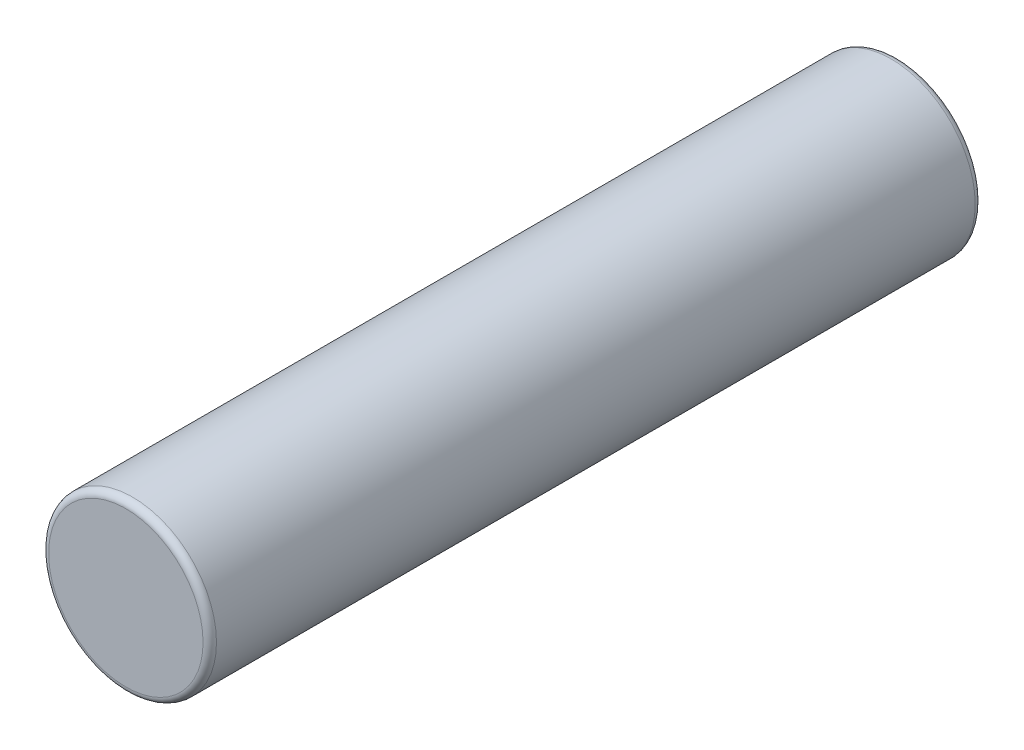
SolidWorks part; units mm, degrees
ref_plane "前视基准面" through (0, 0, 0) normal (0, 0, 1) x (1, 0, 0)
ref_plane "上视基准面" through (0, 0, 0) normal (0, 1, 0) x (1, 0, 0)
ref_plane "右视基准面" through (0, 0, 0) normal (1, 0, 0) x (0, 0, -1)
sketch "草图1" plane through (0, 0, 0) normal (0, 0, 1) x (1, 0, 0)
  circle A0 centre (0, 0) radius 2.5
  dimension "D1" = 5
extrude "凸台-拉伸1" add sketch "草图1" along normal blind 23
fillet "圆角1" radius 0.2 2 edges at (2.5, 0, 0) (2.5, 0, 23)
